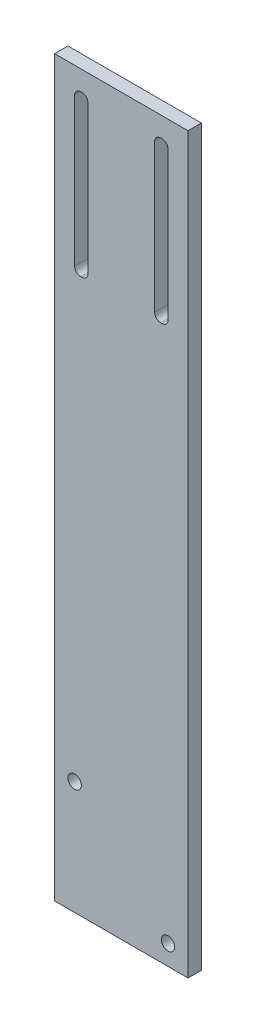
from build123d import *

# Parameters (mm, degrees)
SKETCH1_W           = 100
SKETCH1_H           = 550
BOSS_EXTRUDE1_DEPTH = 10
SKETCH2_R           = 5
CUT_EXTRUDE1_DEPTH  = 10
CUT_EXTRUDE2_DEPTH  = 10


with BuildPart() as part:
    # Sketch1 → Boss-Extrude1 (new body)
    with BuildSketch(Plane.XY):
        Rectangle(SKETCH1_W, SKETCH1_H)
    extrude(amount=BOSS_EXTRUDE1_DEPTH)

    # Sketch2 → Cut-Extrude1 (cut)
    with BuildSketch(Plane.XY.offset(10)):
        with Locations((-35, -190)):
            Circle(SKETCH2_R)
        with Locations((35, -260)):
            Circle(SKETCH2_R)
    extrude(amount=-CUT_EXTRUDE1_DEPTH, mode=Mode.SUBTRACT)

    # Sketch3 → Cut-Extrude2 (cut)
    with BuildSketch(Plane.XY.offset(10)):
        with BuildLine():
            Line((-29.5, 140.099701054), (-30.5, 140.099701054))
            ThreePointArc((-30.5, 140.099701054), (-33.681980515, 141.417720539), (-35, 144.599701054))
            Line((-35, 144.599701054), (-35, 255.599701054))
            ThreePointArc((-35, 255.599701054), (-33.681980515, 258.78168157), (-30.5, 260.099701054))
            Line((-30.5, 260.099701054), (-29.5, 260.099701054))
            ThreePointArc((-29.5, 260.099701054), (-26.318019485, 258.78168157), (-25, 255.599701054))
            Line((-25, 255.599701054), (-25, 144.599701054))
            ThreePointArc((-25, 144.599701054), (-26.318019485, 141.417720539), (-29.5, 140.099701054))
        make_face()
        with BuildLine():
            Line((30.5, 140.099701054), (29.5, 140.099701054))
            ThreePointArc((29.5, 140.099701054), (26.318019485, 141.417720539), (25, 144.599701054))
            Line((25, 144.599701054), (25, 255.599701054))
            ThreePointArc((25, 255.599701054), (26.318019485, 258.78168157), (29.5, 260.099701054))
            Line((29.5, 260.099701054), (30.5, 260.099701054))
            ThreePointArc((30.5, 260.099701054), (33.681980515, 258.78168157), (35, 255.599701054))
            Line((35, 255.599701054), (35, 144.599701054))
            ThreePointArc((35, 144.599701054), (33.681980515, 141.417720539), (30.5, 140.099701054))
        make_face()
    extrude(amount=-CUT_EXTRUDE2_DEPTH, mode=Mode.SUBTRACT)


solid = part.part
